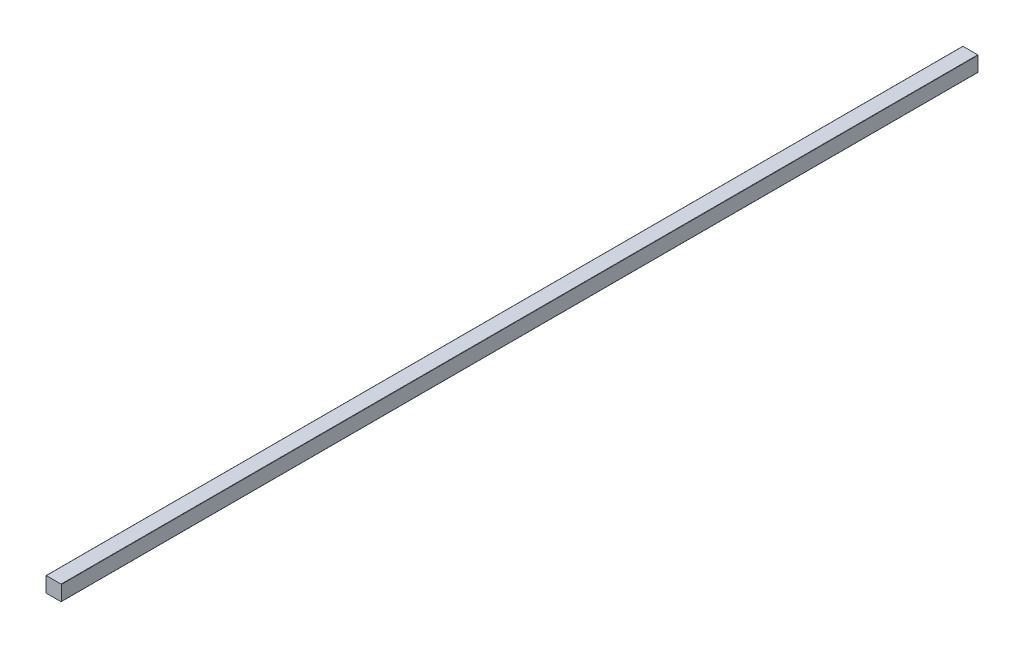
from build123d import *

# Parameters (mm, degrees)
BOSS_EXTRUDE1_DEPTH = 720


with BuildPart() as part:
    # Sketch1 → Boss-Extrude1 (new, symmetric)
    with BuildSketch(Plane.XY):
        with BuildLine():
            Line((-11.5, -12), (11.5, -12))
            ThreePointArc((11.5, -12), (11.853553391, -11.853553391), (12, -11.5))
            Line((12, -11.5), (12, 11.5))
            ThreePointArc((12, 11.5), (11.853553391, 11.853553391), (11.5, 12))
            Line((11.5, 12), (-11.5, 12))
            ThreePointArc((-11.5, 12), (-11.853553391, 11.853553391), (-12, 11.5))
            Line((-12, 11.5), (-12, -11.5))
            ThreePointArc((-12, -11.5), (-11.853553391, -11.853553391), (-11.5, -12))
        make_face()
    extrude(amount=BOSS_EXTRUDE1_DEPTH, both=True)


solid = part.part
